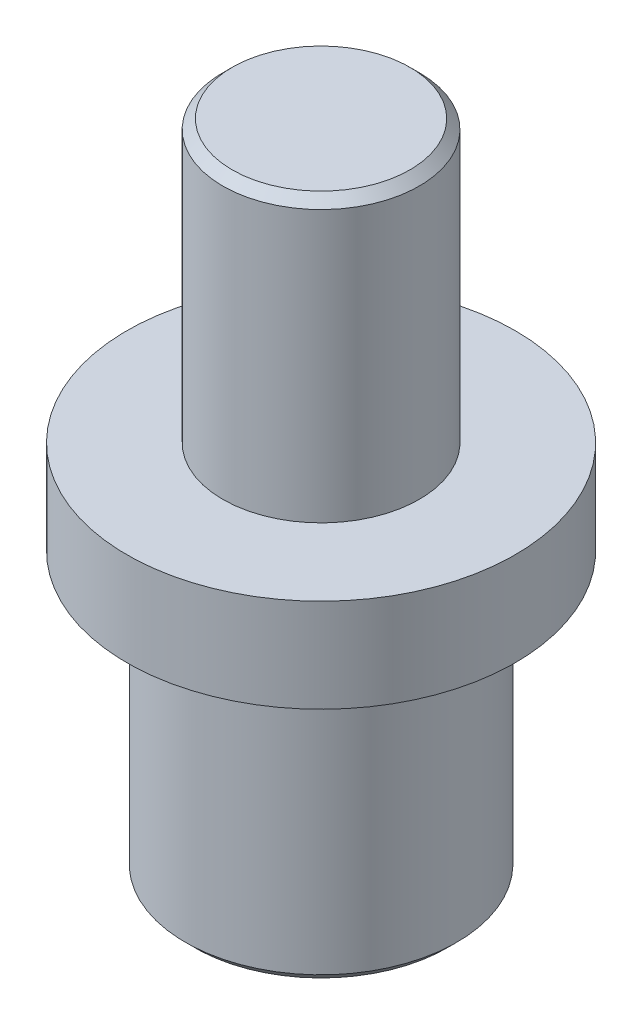
SolidWorks part; units mm, degrees
material "1023 碳钢板 (SS)"
ref_plane "Front Plane" through (0, 0, 0) normal (0, 0, 1) x (1, 0, 0)
ref_plane "Top Plane" through (0, 0, 0) normal (0, 1, 0) x (1, 0, 0)
ref_plane "Right Plane" through (0, 0, 0) normal (1, 0, 0) x (0, 0, -1)
sketch "Sketch1" plane through (0, 0, 0) normal (0, 0, 1) x (1, 0, 0)
  line L0 (0, 0) -> (0, 14)
  line L1 (0, 0) -> (2.9, 0)
  line L2 (2.9, 0) -> (2.9, 6)
  line L3 (2.9, 6) -> (4.15, 6)
  line L4 (4.15, 6) -> (4.15, 8)
  line L5 (4.15, 8) -> (2.1, 8)
  line L6 (2.1, 8) -> (2.1, 14)
  line L7 (2.1, 14) -> (0, 14)
  dimension "D1" = 2.9
  dimension "D2" = 4.15
  dimension "D3" = 2.1
  dimension "D4" = 6
  dimension "D5" = 2
  dimension "D6" = 6
revolve "Revolve1" add sketch "Sketch1" angle 360 about L0
chamfer "Chamfer1" distance 0.2 angle 45 2 edges at (0, 0, -2.9) (0, 14, -2.1)
